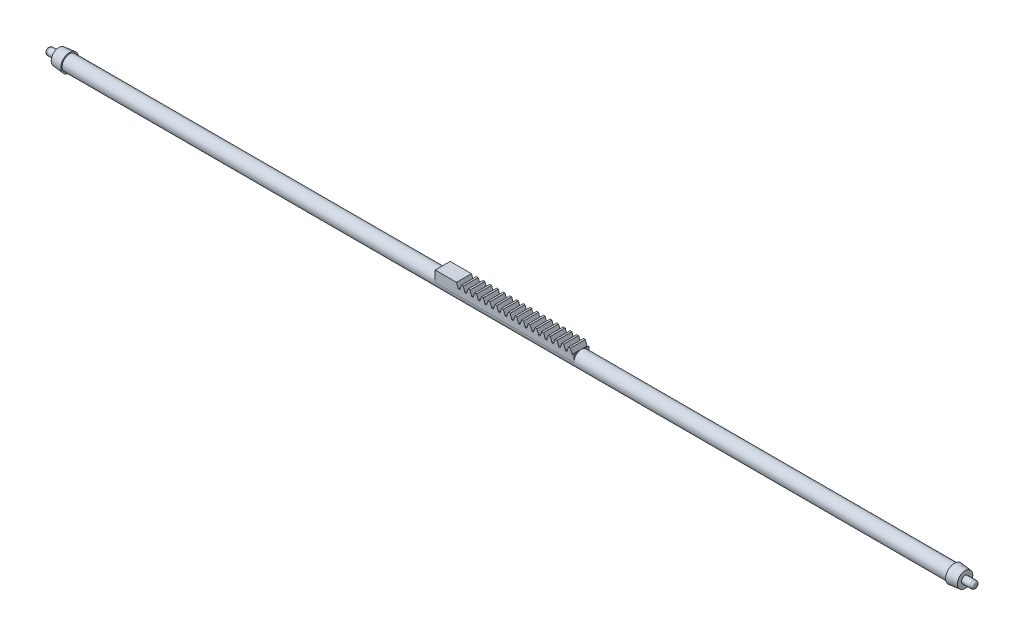
SolidWorks part; units mm, degrees
ref_plane "Front Plane" through (0, 0, 0) normal (0, 0, 1) x (1, 0, 0)
ref_plane "Top Plane" through (0, 0, 0) normal (0, 1, 0) x (1, 0, 0)
ref_plane "Right Plane" through (0, 0, 0) normal (1, 0, 0) x (0, 0, -1)
sketch "Sketch1" plane through (0, 0, 0) normal (0, 0, 1) x (1, 0, 0)
  line L1 (0, 0) -> (13, 0)
  line L2 (0, 0) -> (0, 1)
  line L3 (0, 1) -> (13, 1)
  line L4 (13, 0) -> (13, 1)
  dimension "H0" = 1
  dimension "L" = 13
extrude "Boss-Extrude1" add sketch "Sketch1" along normal blind 1.4
sketch "Sketch2" plane through (0, 0, 1.4) normal (0, 0, 1) x (1, 0, 0)
  line L0 (2, 1) -> (2.1638, 0.55)
  line L1 (13, 1) -> (0, 1) construction
  line L2 (2.1638, 0.55) -> (2.296, 0.55)
  line L3 (2.296, 0.55) -> (2.4597, 1)
  line L4 (2.4597, 1) -> (2, 1)
  line L5 (0, 0.8) -> (13, 0.8) construction
  line L6 (0, 1) -> (0, 0) construction
  line L7 (13, 0) -> (13, 1) construction
  line L9 (2.628, 1) -> (2.7918, 0.55) construction
  line L10 (2.7918, 0.55) -> (2.296, 0.55) construction
  line L12 (2.628, 1) -> (2.4597, 1) construction
  point P12 (2.0728, 0.8)
  point P13 (2.387, 0.8)
  point P14 (2.7008, 0.8)
extrude "Cut-Extrude1" cut sketch "Sketch2" against normal through all
pattern_linear "LPattern1" count 18 spacing 0.628 along (1, 0, 0) of "Cut-Extrude1"
sketch "Sketch3" plane through (0, 0, 0) normal (-1, 0, 0) x (0, 0, 1)
  line L0 (1.4, 0) -> (0, 0) construction
  circle A0 centre (0.7, 0) radius 0.7
extrude "Boss-Extrude2" add sketch "Sketch3" along normal blind 35
sketch "Sketch4" plane through (0, 0, 0) normal (1, 0, 0) x (0, 0, -1)
  line L0 (-1.4, 0) -> (0, 0) construction
  line L1 (0, 0) -> (-1.4, 0)
  arc A0 (-1.4, 0) -> (0, 0) centre (-0.7, 0) ccw
extrude "Boss-Extrude3" add sketch "Sketch4" along normal up to surface (13 mm away) up to face at (13, 0.3135, 0.7)
sketch "Sketch5" plane through (13, 0, 0) normal (1, 0, 0) x (0, 0, -1)
  circle A0 centre (-0.7, 0) radius 0.7
extrude "Boss-Extrude4" add sketch "Sketch5" along normal blind 35
sketch "Sketch6" plane through (48, 0, 0) normal (1, 0, 0) x (0, 0, -1)
  circle A0 centre (-0.7, 0) radius 0.8293
extrude "Boss-Extrude5" add sketch "Sketch6" along normal blind 1 draft 6
sketch "Sketch7" plane through (49, 0, 0) normal (1, 0, 0) x (0, 0, -1)
  circle A0 centre (-0.7, 0) radius 0.33
extrude "Boss-Extrude6" add sketch "Sketch7" along normal blind 1
fillet "Fillet1" radius 0.2 1 edges at (50, 0, 0.37)
ref_plane "Plane1" through (6.5, 0, 0) normal (-1, 0, 0) x (0, 0, 1)
mirror "Mirror1" about plane through (6.5, 0, 0) normal (-1, 0, 0) of "Fillet1", "Boss-Extrude6", "Boss-Extrude5"
equation "\"D3@LPattern1\"= \"P@Sketch2\""
